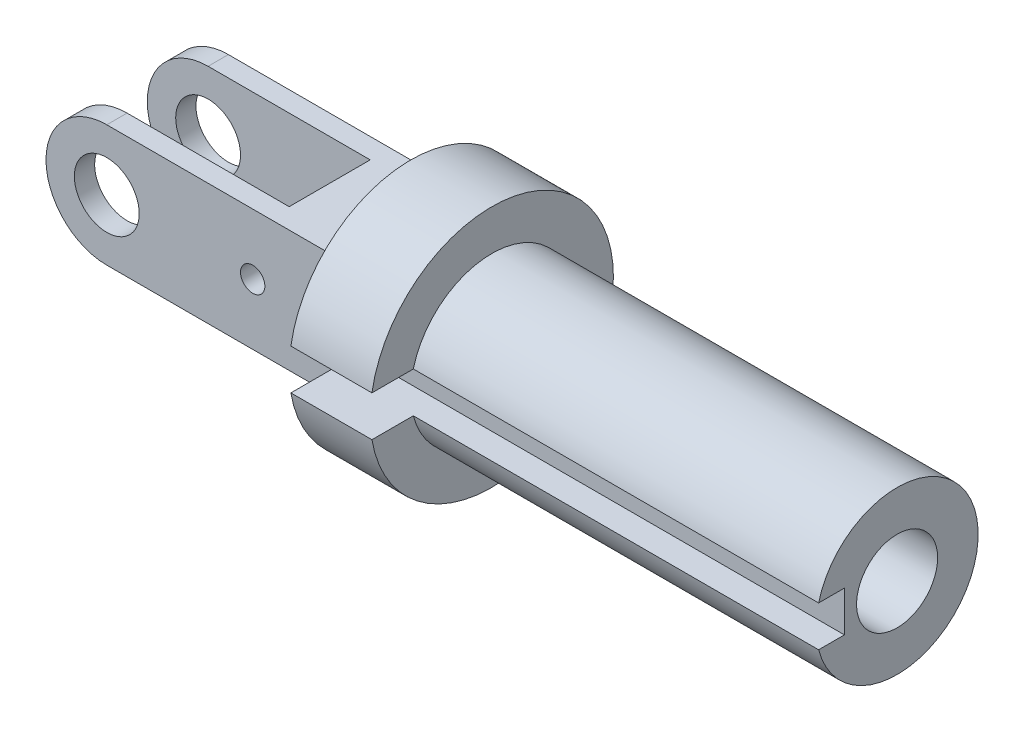
SolidWorks part; units mm, degrees
ref_plane "Front Plane" through (0, 0, 0) normal (0, 0, 1) x (1, 0, 0)
ref_plane "Top Plane" through (0, 0, 0) normal (0, 1, 0) x (1, 0, 0)
ref_plane "Right Plane" through (0, 0, 0) normal (1, 0, 0) x (0, 0, -1)
sketch "Sketch1" plane through (0, 0, 0) normal (0, 0, 1) x (1, 0, 0)
  line L0 (0, -60.0721) -> (0, 2943.5314) construction
  line L1 (0, 0) -> (0, 1.5)
  line L2 (0, 1.5) -> (1, 1.5)
  line L3 (1, 1.5) -> (1, 1)
  line L4 (1, 1) -> (6, 1)
  line L5 (6, 1) -> (6, 0)
  line L6 (0.1244, 0) -> (3003.7278, 0) construction
  line L7 (0, 0) -> (6, 0)
  point P8 (1, 1.25)
  dimension "D1" = 1
  dimension "D2" = 5
  dimension "D3" = 3
  dimension "D4" = 2
revolve "Revolve1" add sketch "Sketch1" angle 360 about L6
sketch "Sketch2" plane through (0, 0, 0) normal (0, 0, 1) x (1, 0, 0)
  line L0 (0, 0) -> (-50000, 0) construction
  line L1 (0, 0.75) -> (0, -0.75)
  line L2 (0, 1.5) -> (0, -1.5) construction
  line L3 (0, -0.75) -> (-3, -0.75)
  line L4 (0, 0) -> (0, 50000) construction
  line L5 (0, 0.75) -> (-3, 0.75)
  arc A0 (-3, -0.75) -> (-3, 0.75) centre (-3, 0) cw
  circle A1 centre (-3, 0) radius 0.4
  point P9 (0, 0)
  dimension "D1" = 0.75
  dimension "D3" = 0.8
  dimension "D2" = 3
extrude "Boss-Extrude1" add sketch "Sketch2" along normal mid plane 1.5
sketch "Sketch3" plane through (0, 0, 0) normal (0, 0, 1) x (1, 0, 0)
  line L0 (-1, 0.75) -> (-1, -0.75)
  line L1 (0, 0.75) -> (-3, 0.75) construction
  line L2 (-3, -0.75) -> (0, -0.75) construction
  line L3 (-1, -0.75) -> (-3, -0.75)
  line L4 (-3, 0.75) -> (-1, 0.75)
  line L5 (0, 1.5) -> (0, -1.5) construction
  arc A0 (-3, -0.75) -> (-3, 0.75) centre (-3, 0) cw
  dimension "D1" = 1
extrude "Cut-Extrude1" cut sketch "Sketch3" against normal mid plane 1
sketch "Sketch4" plane through (6, 0, 0) normal (1, 0, 0) x (0, 0, -1)
  circle A0 centre (0, 0) radius 0.5
extrude "Cut-Extrude2" cut sketch "Sketch4" against normal blind 6
sketch "Sketch5" plane through (6, 0, 0) normal (1, 0, 0) x (0, 0, -1)
  line L0 (-0.65, 0.25) -> (-0.65, -0.25)
  line L1 (-1.8188, -0.25) -> (1.8188, -0.25)
  line L2 (-1.8188, -0.25) -> (-1.8188, 0.25)
  line L3 (-1.8188, 0.25) -> (1.8188, 0.25)
  line L4 (1.8188, -0.25) -> (1.8188, 0.25)
  line L5 (-1.8188, -0.25) -> (1.8188, 0.25) construction
  line L6 (-1.8188, 0.25) -> (1.8188, -0.25) construction
  point P0 (0, 0)
  circle M7 centre (0, 0) radius 1
  dimension "D1" = 0.65
  dimension "D2" = 0.5
extrude "Cut-Extrude4" cut sketch "Sketch5" against normal blind 6 contours L3 L1 L0 M7 | L3 L2 L1 M7
sketch "Sketch6" plane through (0, 0, 0.75) normal (0, 0, 1) x (1, 0, 0)
  line L0 (0, 1.5) -> (0, -1.5) construction
  circle A0 centre (-1.2, 0) radius 0.15
  dimension "D1" = 0.3
  dimension "D2" = 1.2
extrude "Cut-Extrude5" cut sketch "Sketch6" against normal blind 1
